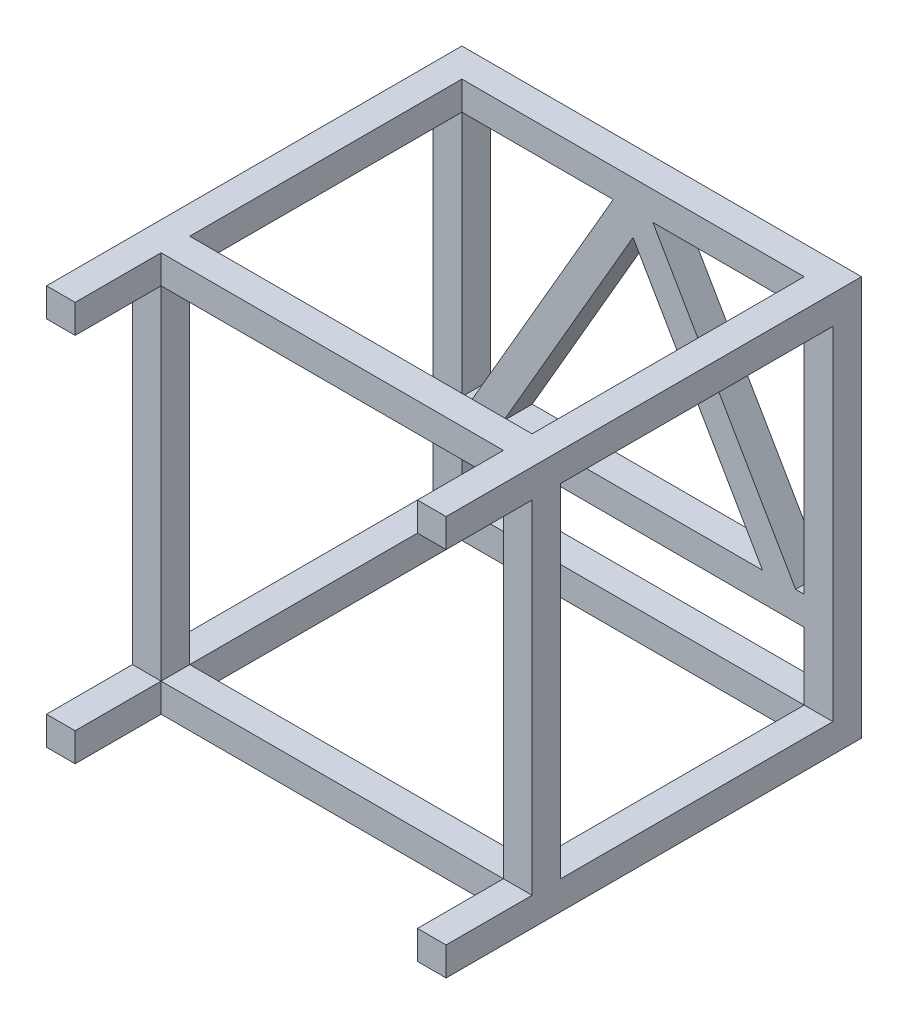
from build123d import *

# Parameters (mm, degrees)
SKETCH1_W           = 1395
SKETCH1_H           = 1395
SKETCH1_W_2         = 1195
SKETCH1_H_2         = 235
BOSS_EXTRUDE1_DEPTH = 100
SKETCH2_W           = 100
SKETCH2_H           = 100
BOSS_EXTRUDE2_DEPTH = 1350
SKETCH3_W           = 100
SKETCH3_H           = 100
BOSS_EXTRUDE3_DEPTH = 1200
SKETCH4_W           = 100
SKETCH4_H           = 100
BOSS_EXTRUDE4_DEPTH = 1200


with BuildPart() as part:
    # Sketch1 → Boss-Extrude1 (new body)
    with BuildSketch(Plane.XY):
        with Locations((697.5, 697.5)):
            Rectangle(SKETCH1_W, SKETCH1_H)
        with Locations((697.5, 217.5)):
            Rectangle(SKETCH1_W_2, SKETCH1_H_2, mode=Mode.SUBTRACT)
        Polygon((100, 1295), (628.279155036, 1295), (130, 435), (100, 435), align=None, mode=Mode.SUBTRACT)
        Polygon((766.720844964, 1295), (1265, 435), (1295, 435), (1295, 1295), align=None, mode=Mode.SUBTRACT)
        Polygon((697.5, 1215), (1149.42760573, 435), (245.57239427, 435), align=None, mode=Mode.SUBTRACT)
    extrude(amount=BOSS_EXTRUDE1_DEPTH)

    # Sketch2 → Boss-Extrude2 (add)
    with BuildSketch(Plane.XY.offset(100)):
        with Locations((50, 1345)):
            Rectangle(SKETCH2_W, SKETCH2_H)
        with Locations((1345, 1345)):
            Rectangle(SKETCH2_W, SKETCH2_H)
        with Locations((50, 50)):
            Rectangle(SKETCH2_W, SKETCH2_H)
        with Locations((1345, 50)):
            Rectangle(SKETCH2_W, SKETCH2_H)
    extrude(amount=BOSS_EXTRUDE2_DEPTH)

    # Sketch3 → Boss-Extrude3 (add)
    with BuildSketch(Plane(origin=(100, 0, 0), x_dir=(0, 0, -1), z_dir=(1, 0, 0))):
        with Locations((-1100, 50)):
            Rectangle(SKETCH3_W, SKETCH3_H)
        with Locations((-1100, 1345)):
            Rectangle(SKETCH3_W, SKETCH3_H)
    extrude(amount=BOSS_EXTRUDE3_DEPTH)

    # Sketch4 → Boss-Extrude4 (add)
    with BuildSketch(Plane(origin=(0, 100, 0), x_dir=(1, 0, 0), z_dir=(0, 1, 0))):
        with Locations((50, -1100)):
            Rectangle(SKETCH4_W, SKETCH4_H)
        with Locations((1345, -1100)):
            Rectangle(SKETCH4_W, SKETCH4_H)
    extrude(amount=BOSS_EXTRUDE4_DEPTH)


solid = part.part
